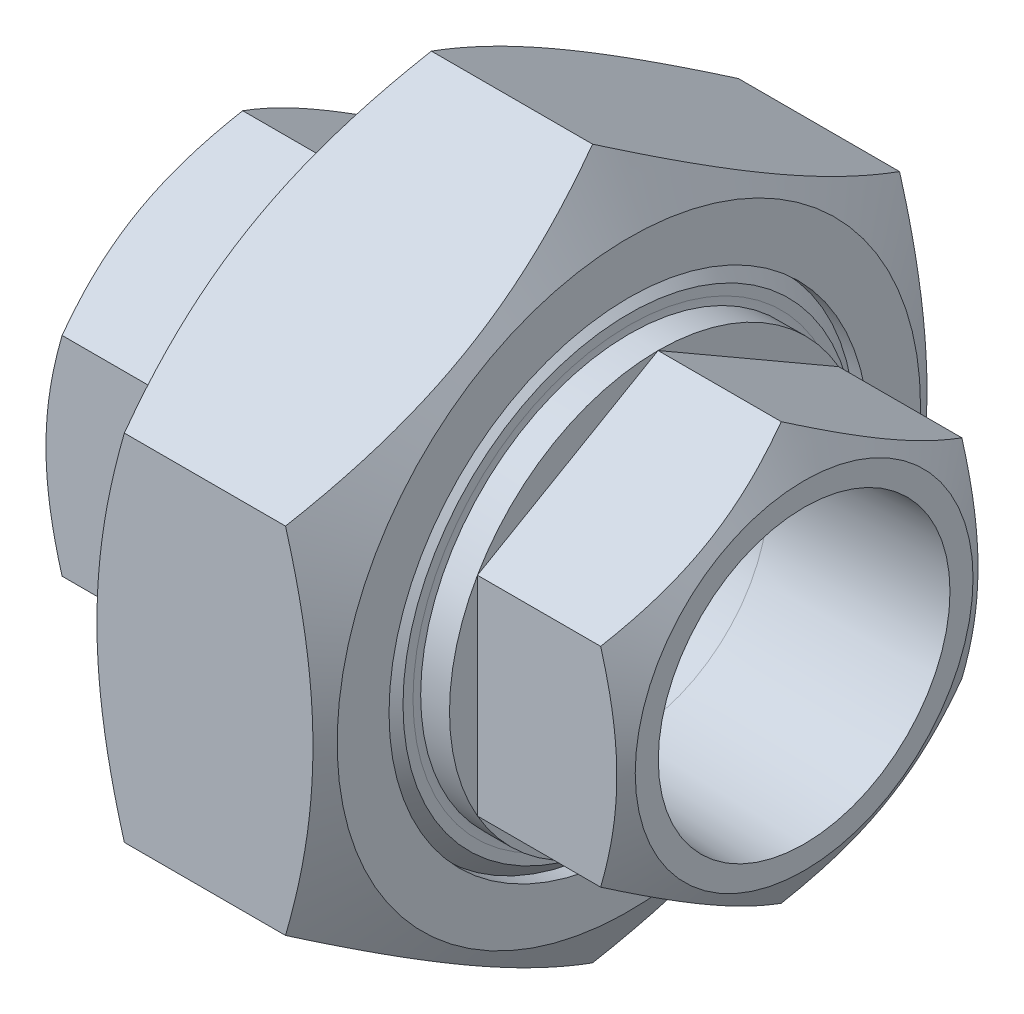
from build123d import *

# Parameters (mm, degrees)
CHAMFER_1_SIZE           = 1.387
CUT_EXTRUDE_START        = -14.5
SKETCH_4_R               = 23.805
CUT_EXTRUDE_1_DEPTH      = 14.5
SKETCH_5_OUTSIDE_W       = 135.604
SKETCH_5_OUTSIDE_H       = 135.604
SKETCH_5_OUTSIDE_R       = 16.767
CUT_EXTRUDE_2_DEPTH      = 11.6
CUT_EXTRUDE_2_DRAFT      = -60
SKETCH_8_R               = 38.709
CUT_EXTRUDE_3_DEPTH      = 65.226413569
SKETCH_10_OUTSIDE_W      = 119.53
SKETCH_10_OUTSIDE_H      = 128.96
SKETCH_10_OUTSIDE_R      = 28.951662261
CUT_EXTRUDE_4_DEPTH      = 10
CUT_EXTRUDE_4_DRAFT      = -60
MIRROR_7_COPY_1_SKETCH_W = 135.604
MIRROR_7_COPY_1_SKETCH_H = 135.604
MIRROR_7_COPY_1_SKETCH_R = 16.767
MIRROR_7_COPY_1_DEPTH    = 11.6
MIRROR_7_COPY_1_DRAFT    = -60
MIRROR_7_COPY_2_SKETCH_W = 119.53
MIRROR_7_COPY_2_SKETCH_H = 128.96
MIRROR_7_COPY_2_SKETCH_R = 28.951662261
MIRROR_7_COPY_2_DEPTH    = 10
MIRROR_7_COPY_2_DRAFT    = -60


with BuildPart() as part:
    # 草图1 → 旋转1 (revolve)
    with BuildSketch(Plane.XY, mode=Mode.PRIVATE) as revolve_1_sk:
        Polygon((29, 20.7), (11.6, 20.7), (11.6, 23.805), (0, 23.805), (0, 27.324), (-11.6, 27.324), (-11.6, 20.7), (-29, 20.7), (-29, 14.477621389), (-11.6, 13.87), (11.6, 13.87), (29, 14.477621389), align=None)
    revolve(revolve_1_sk.sketch.rotate(Axis((0, 0, 0), (1, 0, 0)), 90), axis=Axis((0, 0, 0), (1, 0, 0)))

    # 倒角1
    chamfer_1_edges = [part.edges().sort_by_distance(p)[0] for p in [
        (-11.6, 0, -27.324),
        (11.6, 0, -23.805),
    ]]
    chamfer(chamfer_1_edges, length=CHAMFER_1_SIZE)

    # 草图3 → 旋转2 (revolve)
    with BuildSketch(Plane.XY, mode=Mode.PRIVATE) as revolve_2_sk:
        Polygon((-11.6, 27.324), (-11.6, 35.19), (11.6, 35.19), (11.6, 23.805), (0, 23.805), (0, 27.324), align=None)
    revolve(revolve_2_sk.sketch.rotate(Axis((0, 0, 0), (1, 0, 0)), 90), axis=Axis((0, 0, 0), (1, 0, 0)))

    # 草图4 → 切除-拉伸1 (cut)
    with BuildSketch(Plane(origin=(29, 0, 0), x_dir=(0, 0, -1), z_dir=(1, 0, 0)).offset(CUT_EXTRUDE_START)):
        with Locations(Location((0, 0, 0), (0, 0, 180))):
            Circle(SKETCH_4_R)
        Polygon((0, 20.7), (-17.926725858, 10.35), (-17.926725858, -10.35), (0, -20.7), (17.926725858, -10.35), (17.926725858, 10.35), align=None, mode=Mode.SUBTRACT)
    cut_extrude_1 = extrude(amount=CUT_EXTRUDE_1_DEPTH, mode=Mode.SUBTRACT)


with BuildPart() as cut_extrude_2_tool:
    # 草图5 outside → 切除-拉伸2 (with draft: the straight prism first)
    with BuildSketch(Plane(origin=(29, 0, 0), x_dir=(0, 0, -1), z_dir=(1, 0, 0))):
        Rectangle(SKETCH_5_OUTSIDE_W, SKETCH_5_OUTSIDE_H)
        Circle(SKETCH_5_OUTSIDE_R, mode=Mode.SUBTRACT)
    extrude(amount=-CUT_EXTRUDE_2_DEPTH)
    # 切除-拉伸2: the draft: its side faces are tilted about the plane it starts from
    cut_extrude_2_sides = [cut_extrude_2_tool.faces().sort_by_distance(p)[0] for p in [
        (23.2, -67.802, 0),
        (23.2, 0, -67.802),
        (23.2, 67.802, 0),
        (23.2, 0, 67.802),
        (23.2, 0, 16.767),
    ]]
    draft(cut_extrude_2_sides, Plane(origin=(29, 0, 0), x_dir=(0, 0, -1), z_dir=(1, 0, 0)), CUT_EXTRUDE_2_DRAFT)


with BuildPart() as part_1:
    add(part.part)

    # 切除-拉伸2: cut by cut_extrude_2_tool
    add(cut_extrude_2_tool.part, mode=Mode.SUBTRACT)

    # 草图6 → 旋转3 (revolve)
    with BuildSketch(Plane.XY, mode=Mode.PRIVATE) as revolve_3_sk:
        with BuildLine():
            Line((18.899592609, 14.124907391), (11.6, 14.124907391))
            Line((11.6, 14.124907391), (11.6, 21.4245))
            ThreePointArc((11.6, 21.4245), (13.738001175, 16.262908566), (18.899592609, 14.124907391))
        make_face()
    revolve_3 = revolve(revolve_3_sk.sketch.rotate(Axis((0, 0, 0), (1, 0, 0)), 120), axis=Axis((0, 0, 0), (1, 0, 0)))

    # 草图8 → 切除-拉伸3 (cut, through all)
    with BuildSketch(Plane(origin=(11.6, 0, 0), x_dir=(0, 0, -1), z_dir=(1, 0, 0))):
        Circle(SKETCH_8_R)
        Polygon((0, 35.19), (-30.475433959, 17.595), (-30.475433959, -17.595), (0, -35.19), (30.475433959, -17.595), (30.475433959, 17.595), align=None, mode=Mode.SUBTRACT)
    extrude(amount=-CUT_EXTRUDE_3_DEPTH, mode=Mode.SUBTRACT)


with BuildPart() as cut_extrude_4_tool:
    # 草图10 outside → 切除-拉伸4 (with draft: the straight prism first)
    with BuildSketch(Plane(origin=(11.6, 0, 0), x_dir=(0, 0, -1), z_dir=(1, 0, 0))):
        Rectangle(SKETCH_10_OUTSIDE_W, SKETCH_10_OUTSIDE_H)
        Circle(SKETCH_10_OUTSIDE_R, mode=Mode.SUBTRACT)
    extrude(amount=-CUT_EXTRUDE_4_DEPTH)
    # 切除-拉伸4: the draft: its side faces are tilted about the plane it starts from
    cut_extrude_4_sides = [cut_extrude_4_tool.faces().sort_by_distance(p)[0] for p in [
        (6.6, -64.48, 0),
        (6.6, 0, -59.765),
        (6.6, 64.48, 0),
        (6.6, 0, 59.765),
        (6.6, 0, 28.951662261),
    ]]
    draft(cut_extrude_4_sides, Plane(origin=(11.6, 0, 0), x_dir=(0, 0, -1), z_dir=(1, 0, 0)), CUT_EXTRUDE_4_DRAFT)


with BuildPart() as part_2:
    add(part_1.part)

    # 切除-拉伸4: cut by cut_extrude_4_tool
    add(cut_extrude_4_tool.part, mode=Mode.SUBTRACT)

    # 镜向7: 切除-拉伸1, 旋转3 across plane
    add(cut_extrude_1.mirror(Plane(origin=(0, 0, 0), x_dir=(0, 0, 1), z_dir=(1, 0, 0))), mode=Mode.SUBTRACT)
    add(revolve_3.mirror(Plane(origin=(0, 0, 0), x_dir=(0, 0, 1), z_dir=(1, 0, 0))))


with BuildPart() as mirror_7_copy_1_tool:
    # 镜向7 copy 1 sketch → 镜向7 copy 1 (with draft: the straight prism first)
    with BuildSketch(Plane(origin=(-29, 0, 0), x_dir=(0, 0, -1), z_dir=(-1, 0, 0))):
        Rectangle(MIRROR_7_COPY_1_SKETCH_W, MIRROR_7_COPY_1_SKETCH_H)
        Circle(MIRROR_7_COPY_1_SKETCH_R, mode=Mode.SUBTRACT)
    extrude(amount=-MIRROR_7_COPY_1_DEPTH)
    # 镜向7 copy 1: the draft: its side faces are tilted about the plane it starts from
    mirror_7_copy_1_sides = [mirror_7_copy_1_tool.faces().sort_by_distance(p)[0] for p in [
        (-23.2, -67.802, 0),
        (-23.2, 0, -67.802),
        (-23.2, 67.802, 0),
        (-23.2, 0, 67.802),
        (-23.2, 0, 16.767),
    ]]
    draft(mirror_7_copy_1_sides, Plane(origin=(-29, 0, 0), x_dir=(0, 0, -1), z_dir=(-1, 0, 0)), MIRROR_7_COPY_1_DRAFT)


with BuildPart() as part_3:
    add(part_2.part)

    # 镜向7 copy 1: cut by mirror_7_copy_1_tool
    add(mirror_7_copy_1_tool.part, mode=Mode.SUBTRACT)


with BuildPart() as mirror_7_copy_2_tool:
    # 镜向7 copy 2 sketch → 镜向7 copy 2 (with draft: the straight prism first)
    with BuildSketch(Plane(origin=(-11.6, 0, 0), x_dir=(0, 0, -1), z_dir=(-1, 0, 0))):
        Rectangle(MIRROR_7_COPY_2_SKETCH_W, MIRROR_7_COPY_2_SKETCH_H)
        Circle(MIRROR_7_COPY_2_SKETCH_R, mode=Mode.SUBTRACT)
    extrude(amount=-MIRROR_7_COPY_2_DEPTH)
    # 镜向7 copy 2: the draft: its side faces are tilted about the plane it starts from
    mirror_7_copy_2_sides = [mirror_7_copy_2_tool.faces().sort_by_distance(p)[0] for p in [
        (-6.6, -64.48, 0),
        (-6.6, 0, -59.765),
        (-6.6, 64.48, 0),
        (-6.6, 0, 59.765),
        (-6.6, 0, 28.951662261),
    ]]
    draft(mirror_7_copy_2_sides, Plane(origin=(-11.6, 0, 0), x_dir=(0, 0, -1), z_dir=(-1, 0, 0)), MIRROR_7_COPY_2_DRAFT)


with BuildPart() as part_4:
    add(part_3.part)

    # 镜向7 copy 2: cut by mirror_7_copy_2_tool
    add(mirror_7_copy_2_tool.part, mode=Mode.SUBTRACT)


solid = part_4.part
